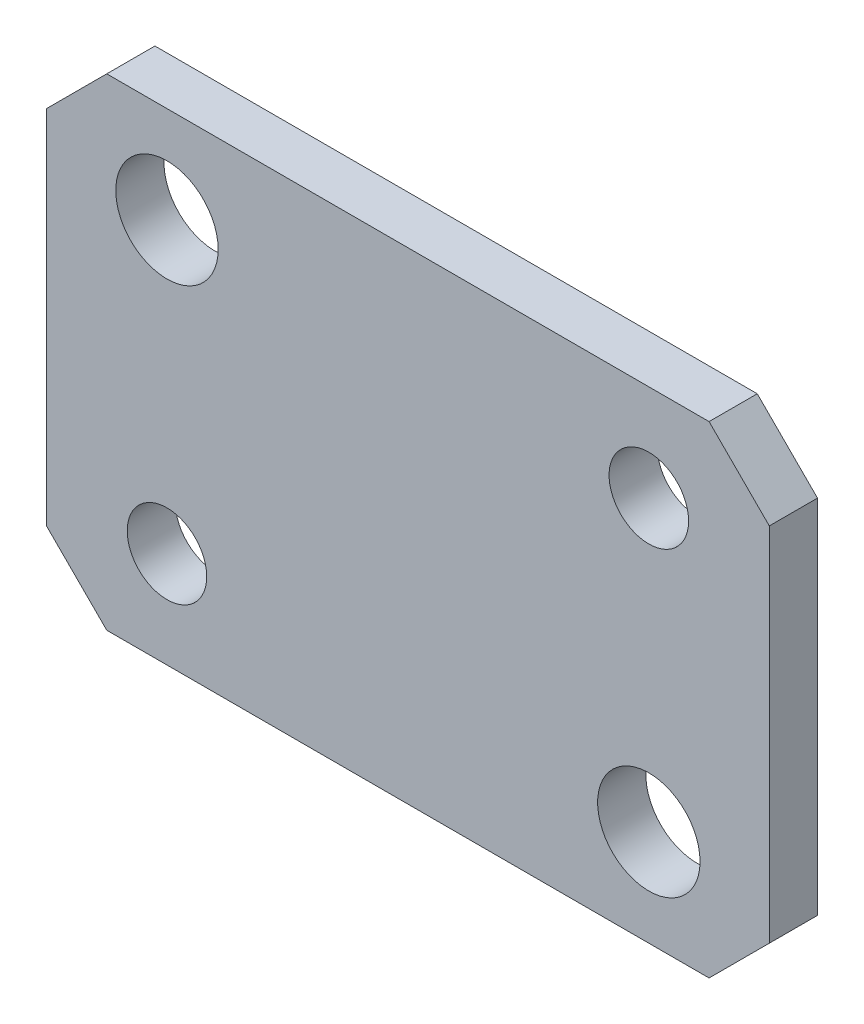
from build123d import *

# Parameters (mm, degrees)
SKETCH1_W           = 60
SKETCH1_H           = 40
SKETCH1_R           = 4.25
SKETCH1_R_2         = 3.3
BOSS_EXTRUDE1_DEPTH = 4
CHAMFER1_SIZE       = 5


with BuildPart() as part:
    # Sketch1 → Boss-Extrude1 (new body)
    with BuildSketch(Plane.XY):
        with Locations((5.009460805, -5.533568905)):
            Rectangle(SKETCH1_W, SKETCH1_H)
        with Locations((-14.990539195, 6.466431095)):
            Circle(SKETCH1_R, mode=Mode.SUBTRACT)
        with Locations((25.009460805, -17.533568905)):
            Circle(SKETCH1_R, mode=Mode.SUBTRACT)
        with Locations((25.009460805, 6.466431095)):
            Circle(SKETCH1_R_2, mode=Mode.SUBTRACT)
        with Locations((-14.990539195, -17.533568905)):
            Circle(SKETCH1_R_2, mode=Mode.SUBTRACT)
    extrude(amount=BOSS_EXTRUDE1_DEPTH)

    # Chamfer1
    chamfer1_edges = [part.edges().sort_by_distance(p)[0] for p in [
        (-24.990539195, 14.466431095, 2),
        (35.009460805, 14.466431095, 2),
        (35.009460805, -25.533568905, 2),
        (-24.990539195, -25.533568905, 2),
    ]]
    chamfer(chamfer1_edges, length=CHAMFER1_SIZE)


solid = part.part
